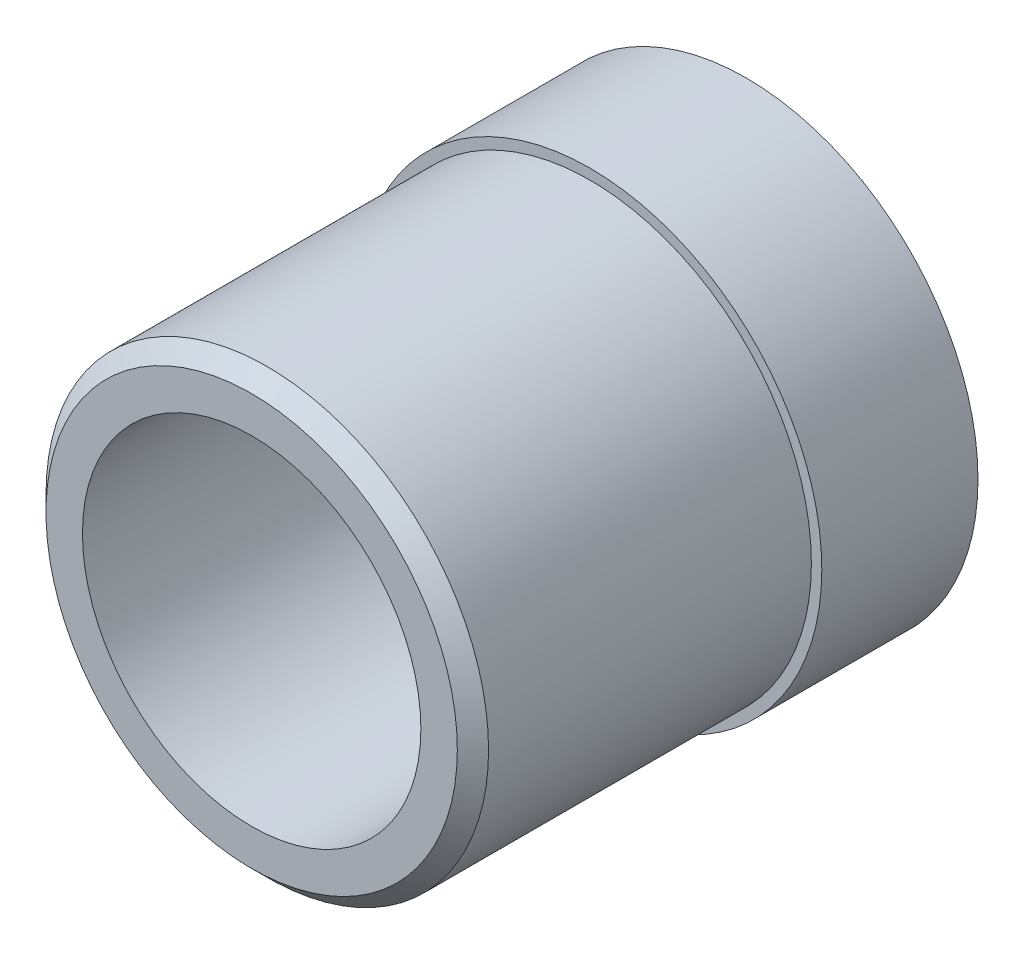
SolidWorks part; units mm, degrees
material "普通碳钢"
ref_plane "前视基准面" through (0, 0, 0) normal (0, 0, 1) x (1, 0, 0)
ref_plane "上视基准面" through (0, 0, 0) normal (0, 1, 0) x (1, 0, 0)
ref_plane "右视基准面" through (0, 0, 0) normal (1, 0, 0) x (0, 0, -1)
sketch "草图1" plane through (0, 0, 0) normal (0, 0, 1) x (1, 0, 0)
  circle A0 centre (0, 0) radius 44.5
  circle A1 centre (0, 0) radius 32.5
  dimension "D1" = 89
  dimension "D2" = 65
extrude "凸台-拉伸1" add sketch "草图1" along normal blind 95
sketch "草图2" plane through (0, 0, 95) normal (0, 0, 1) x (1, 0, 0)
  circle A0 centre (0, 0) radius 42.5
  circle A1 centre (0, 0) radius 44.5
  dimension "D1" = 85
  dimension "D2" = 89
extrude "切除-拉伸1" cut sketch "草图2" against normal blind 65
chamfer "倒角1" distance 3 angle 45 1 edges at (42.5, 0, 95)
